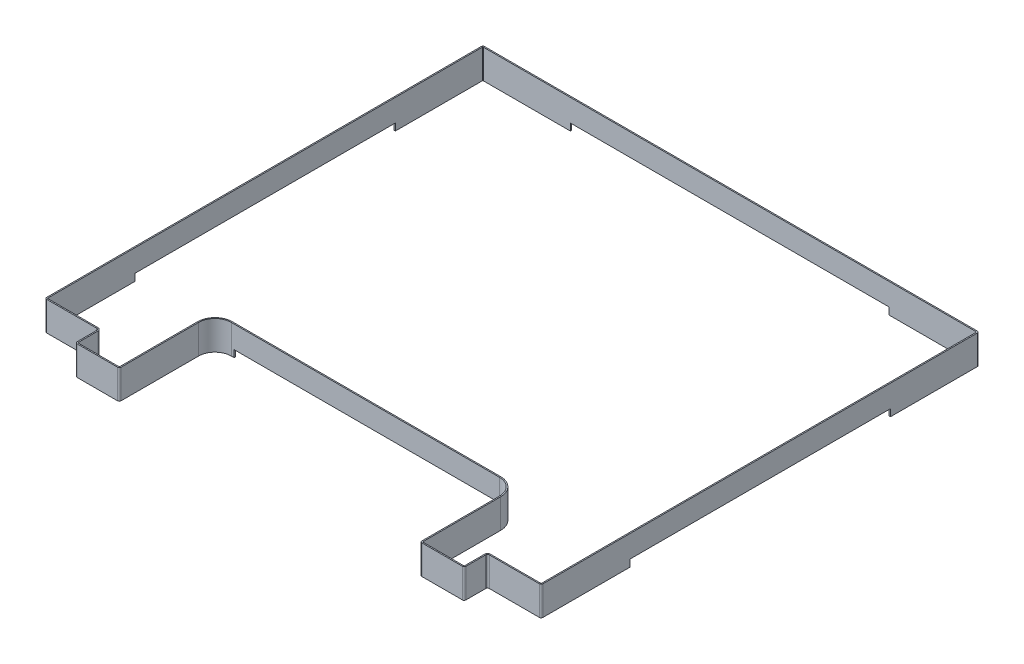
SolidWorks part; units mm, degrees
ref_plane "前视" through (0, 0, 0) normal (0, 0, 1) x (1, 0, 0)
ref_plane "上视" through (0, 0, 0) normal (0, 1, 0) x (1, 0, 0)
ref_plane "右视" through (0, 0, 0) normal (1, 0, 0) x (0, 0, -1)
sketch "草图1" plane through (0, 0, 0) normal (0, 1, 0) x (1, 0, 0)
  line L1 (-333.5, 395.5) -> (333.5, 395.5)
  line L2 (-333.5, 395.5) -> (-333.5, -395.5)
  line L3 (-333.5, -395.5) -> (333.5, -395.5)
  line L4 (333.5, 395.5) -> (333.5, -395.5)
  line L5 (-333.5, 395.5) -> (333.5, -395.5) construction
  line L6 (-333.5, -395.5) -> (333.5, 395.5) construction
  point P0 (0, 0)
  dimension "D1" = 667
  dimension "D2" = 791
extrude "凸台-拉伸1" add sketch "草图1" along normal blind 50
sketch "草图6" plane through (0, 50, 0) normal (0, 1, 0) x (1, 0, 0)
  line L0 (0, 0) -> (0, -181.1931) construction
  line L1 (-333.5, -395.5) -> (333.5, -395.5) construction
  line L2 (-258, -395.5) -> (258, -395.5)
  line L3 (-258, -395.5) -> (-258, -231.5)
  line L4 (-258, -231.5) -> (258, -231.5)
  line L5 (258, -395.5) -> (258, -231.5)
  dimension "D1" = 164
  dimension "D2" = 516
extrude "切除-拉伸1" cut sketch "草图6" against normal through all
sketch "草图4" plane through (333.5, 0, 0) normal (1, 0, 0) x (0, 0, -1)
  line L1 (-395.5, 50) -> (395.5, 50) construction
  line L3 (-355.5, 50) -> (-355.5, 0)
  line L4 (-395.5, 0) -> (395.5, 0) construction
  line L5 (-355.5, 0) -> (395.5, 0)
  line L6 (395.5, 0) -> (395.5, 50)
  line L7 (395.5, 50) -> (-355.5, 50)
  line L8 (-395.5, 50) -> (-395.5, 0) construction
  dimension "D1" = 40
extrude "凸台-拉伸2" add sketch "草图4" along normal blind 92
sketch "草图5" plane through (-333.5, 0, 0) normal (-1, 0, 0) x (0, 0, 1)
  line L2 (355.5, 50) -> (355.5, 0) construction
  line L3 (-395.5, 0) -> (395.5, 0) construction
  line L4 (-395.5, 50) -> (-395.5, 0) construction
  line L5 (-395.5, 50) -> (395.5, 50) construction
  line L8 (355.5, 50) -> (355.5, 0)
  line L9 (-395.5, 0) -> (355.5, 0)
  line L10 (-395.5, 50) -> (-395.5, 0)
  line L11 (-395.5, 50) -> (355.5, 50)
extrude "凸台-拉伸3" add sketch "草图5" along normal blind 92
shell "抽壳2" thickness 2
fillet "圆角1" radius 1 8 edges at (331.5, 25, 393.5) (-260, 25, 393.5) (-331.5, 25, 393.5) (260, 25, 393.5) (423.5, 25, 353.5) (423.5, 25, -393.5) (-423.5, 25, -393.5) (-423.5, 25, 353.5)
fillet "圆角2" radius 3 10 edges at (425.5, 25, 355.5) (425.5, 25, -395.5) (-425.5, 25, -395.5) (-425.5, 25, 355.5) (333.5, 25, 395.5) (-333.5, 25, 395.5) (258, 25, 395.5) (-258, 25, 395.5)
fillet "圆角3" radius 5 2 edges at (331.5, 25, 353.5) (-331.5, 25, 353.5)
fillet "圆角4" radius 28 2 edges at (258, 25, 231.5) (-258, 25, 231.5)
fillet "圆角5" radius 30 2 edges at (-260, 25, 229.5) (260, 25, 229.5)
sketch "草图7" plane through (425.5, 0, 0) normal (1, 0, 0) x (0, 0, -1)
  line L0 (-203.5, 12) -> (243.5, 12)
  line L1 (243.5, 12) -> (243.5, 0)
  line L2 (-352.5, 0) -> (392.5, 0) construction
  line L3 (243.5, 0) -> (-203.5, 0)
  line L4 (-203.5, 0) -> (-203.5, 12)
  line L5 (20, 50) -> (20, -14.7356) construction
  line L6 (392.5, 50) -> (-352.5, 50) construction
  dimension "D2" = 12
  dimension "D3" = 447
extrude "切除-拉伸2" cut sketch "草图7" against normal blind 2
sketch "草图8" plane through (-425.5, 0, 0) normal (-1, 0, 0) x (0, 0, 1)
  line L0 (203.5, 12) -> (203.5, 0) construction
  line L1 (-243.5, 12) -> (203.5, 12) construction
  line L2 (-243.5, 0) -> (-243.5, 12) construction
  line L3 (-392.5, 0) -> (352.5, 0) construction
  line L4 (203.5, 12) -> (203.5, 0)
  line L5 (-243.5, 12) -> (203.5, 12)
  line L6 (-243.5, 0) -> (-243.5, 12)
  line L7 (-243.5, 0) -> (203.5, 0)
extrude "切除-拉伸3" cut sketch "草图8" against normal blind 2
sketch "草图9" plane through (0, 0, -395.5) normal (0, 0, -1) x (-1, 0, 0)
  line L0 (0, 0) -> (0, 114.9427) construction
  line L2 (-273.5, 12) -> (273.5, 12)
  line L3 (-273.5, 12) -> (-273.5, 0)
  line L4 (-273.5, 0) -> (273.5, 0)
  line L5 (273.5, 12) -> (273.5, 0)
  line L6 (-422.5, 0) -> (422.5, 0) construction
  dimension "D1" = 547
  dimension "D2" = 12
extrude "切除-拉伸4" cut sketch "草图9" against normal blind 2
sketch "草图10" plane through (0, 0, 231.5) normal (0, 0, 1) x (1, 0, 0)
  line L0 (0, 0) -> (0, 96.0861) construction
  line L1 (230, 0) -> (-230, 0) construction
  line L2 (-225, 0) -> (225, 0)
  line L3 (-225, 0) -> (-225, 12)
  line L4 (-225, 12) -> (225, 12)
  line L5 (225, 0) -> (225, 12)
  dimension "D1" = 12
  dimension "D2" = 450
extrude "切除-拉伸5" cut sketch "草图10" against normal mid plane 100
